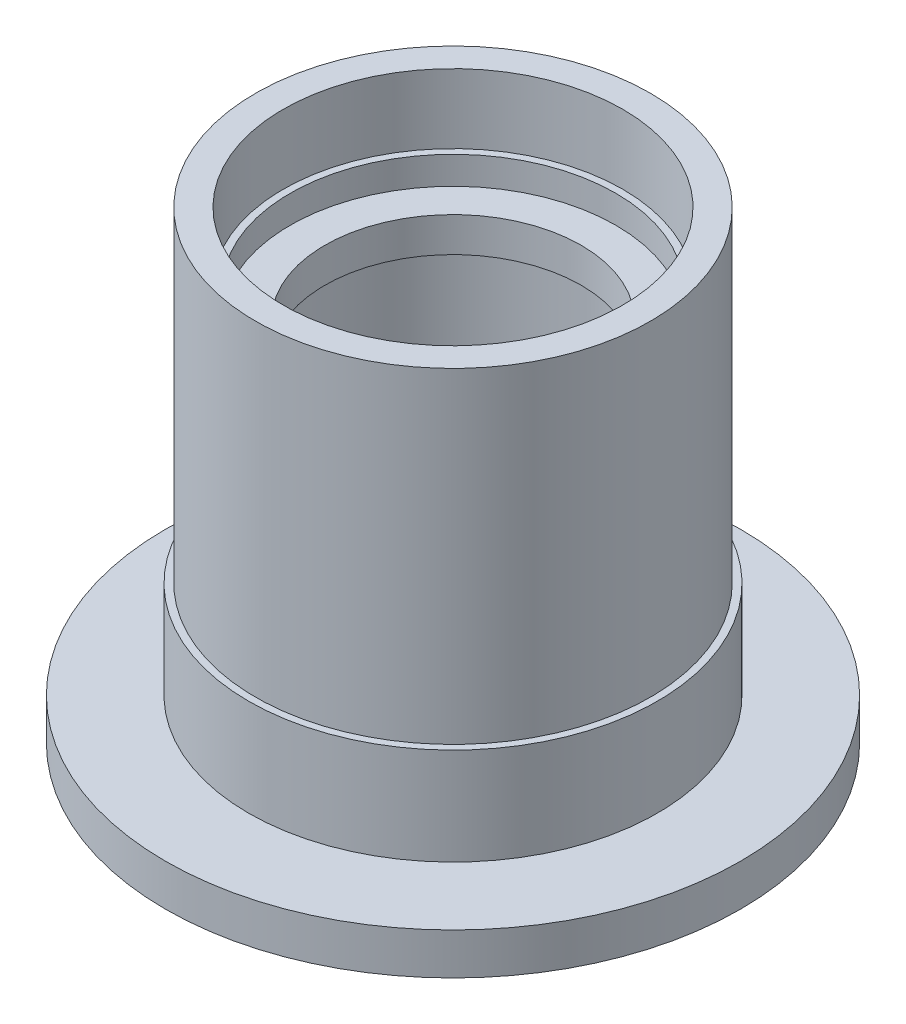
from build123d import *


with BuildPart() as part:
    # 草图1 → 旋转1 (revolve)
    with BuildSketch(Plane.XY, mode=Mode.PRIVATE) as revolve_1_sk:
        Polygon((-23.5, 57), (-23.5, 53), (-18.5, 53), (-18.5, 48), (-21.5, 48), (-21.5, 24), (-23.5, 24), (-23.5, 0), (-41.5, 0), (-41.5, 6), (-29.5, 6), (-29.5, 20), (-28.5, 20), (-28.5, 67), (-24.5, 67), (-24.5, 57), align=None)
    revolve(revolve_1_sk.sketch.rotate(Axis((0, 0, 0), (0, 1, 0)), 270), axis=Axis((0, 0, 0), (0, 1, 0)))


solid = part.part
